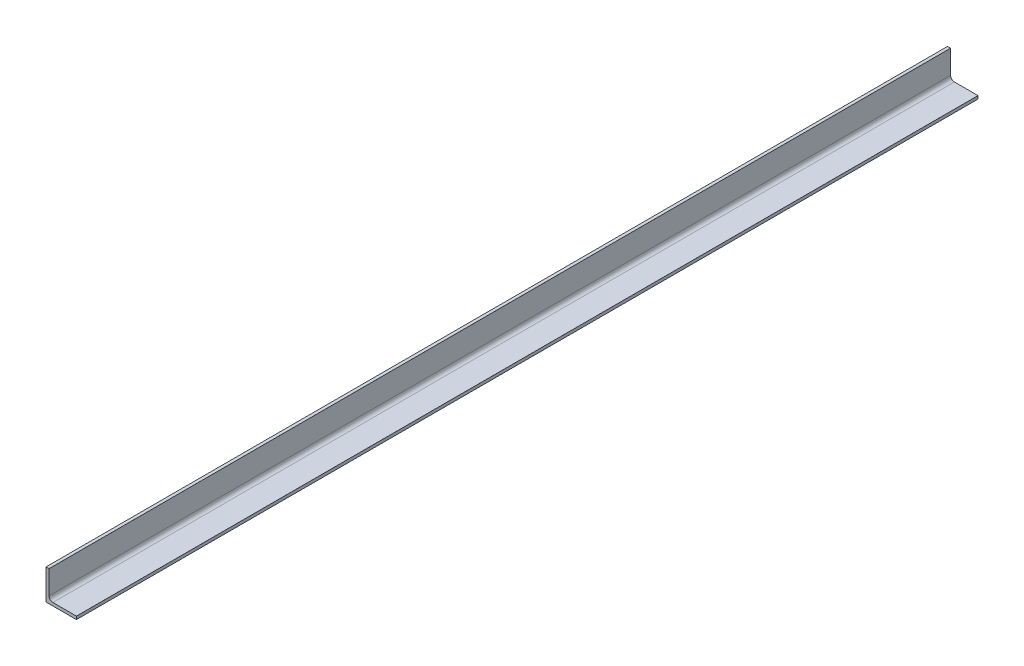
from build123d import *

# Parameters (mm, degrees)
EXTRUDE_1_DEPTH = 1185


with BuildPart() as part:
    # 草图1 → 拉伸1 (new body)
    with BuildSketch(Plane.XY):
        with BuildLine():
            Line((0, 0), (0, 40))
            Line((0, 40), (3.99, 40))
            ThreePointArc((3.99, 40), (3.997071068, 39.997071068), (4, 39.99))
            Line((4, 39.99), (4, 9))
            ThreePointArc((4, 9), (5.464466094, 5.464466094), (9, 4))
            Line((9, 4), (39.99, 4))
            ThreePointArc((39.99, 4), (39.997071068, 3.997071068), (40, 3.99))
            Line((40, 3.99), (40, 0))
            Line((40, 0), (0, 0))
        make_face()
    extrude(amount=EXTRUDE_1_DEPTH)


solid = part.part
